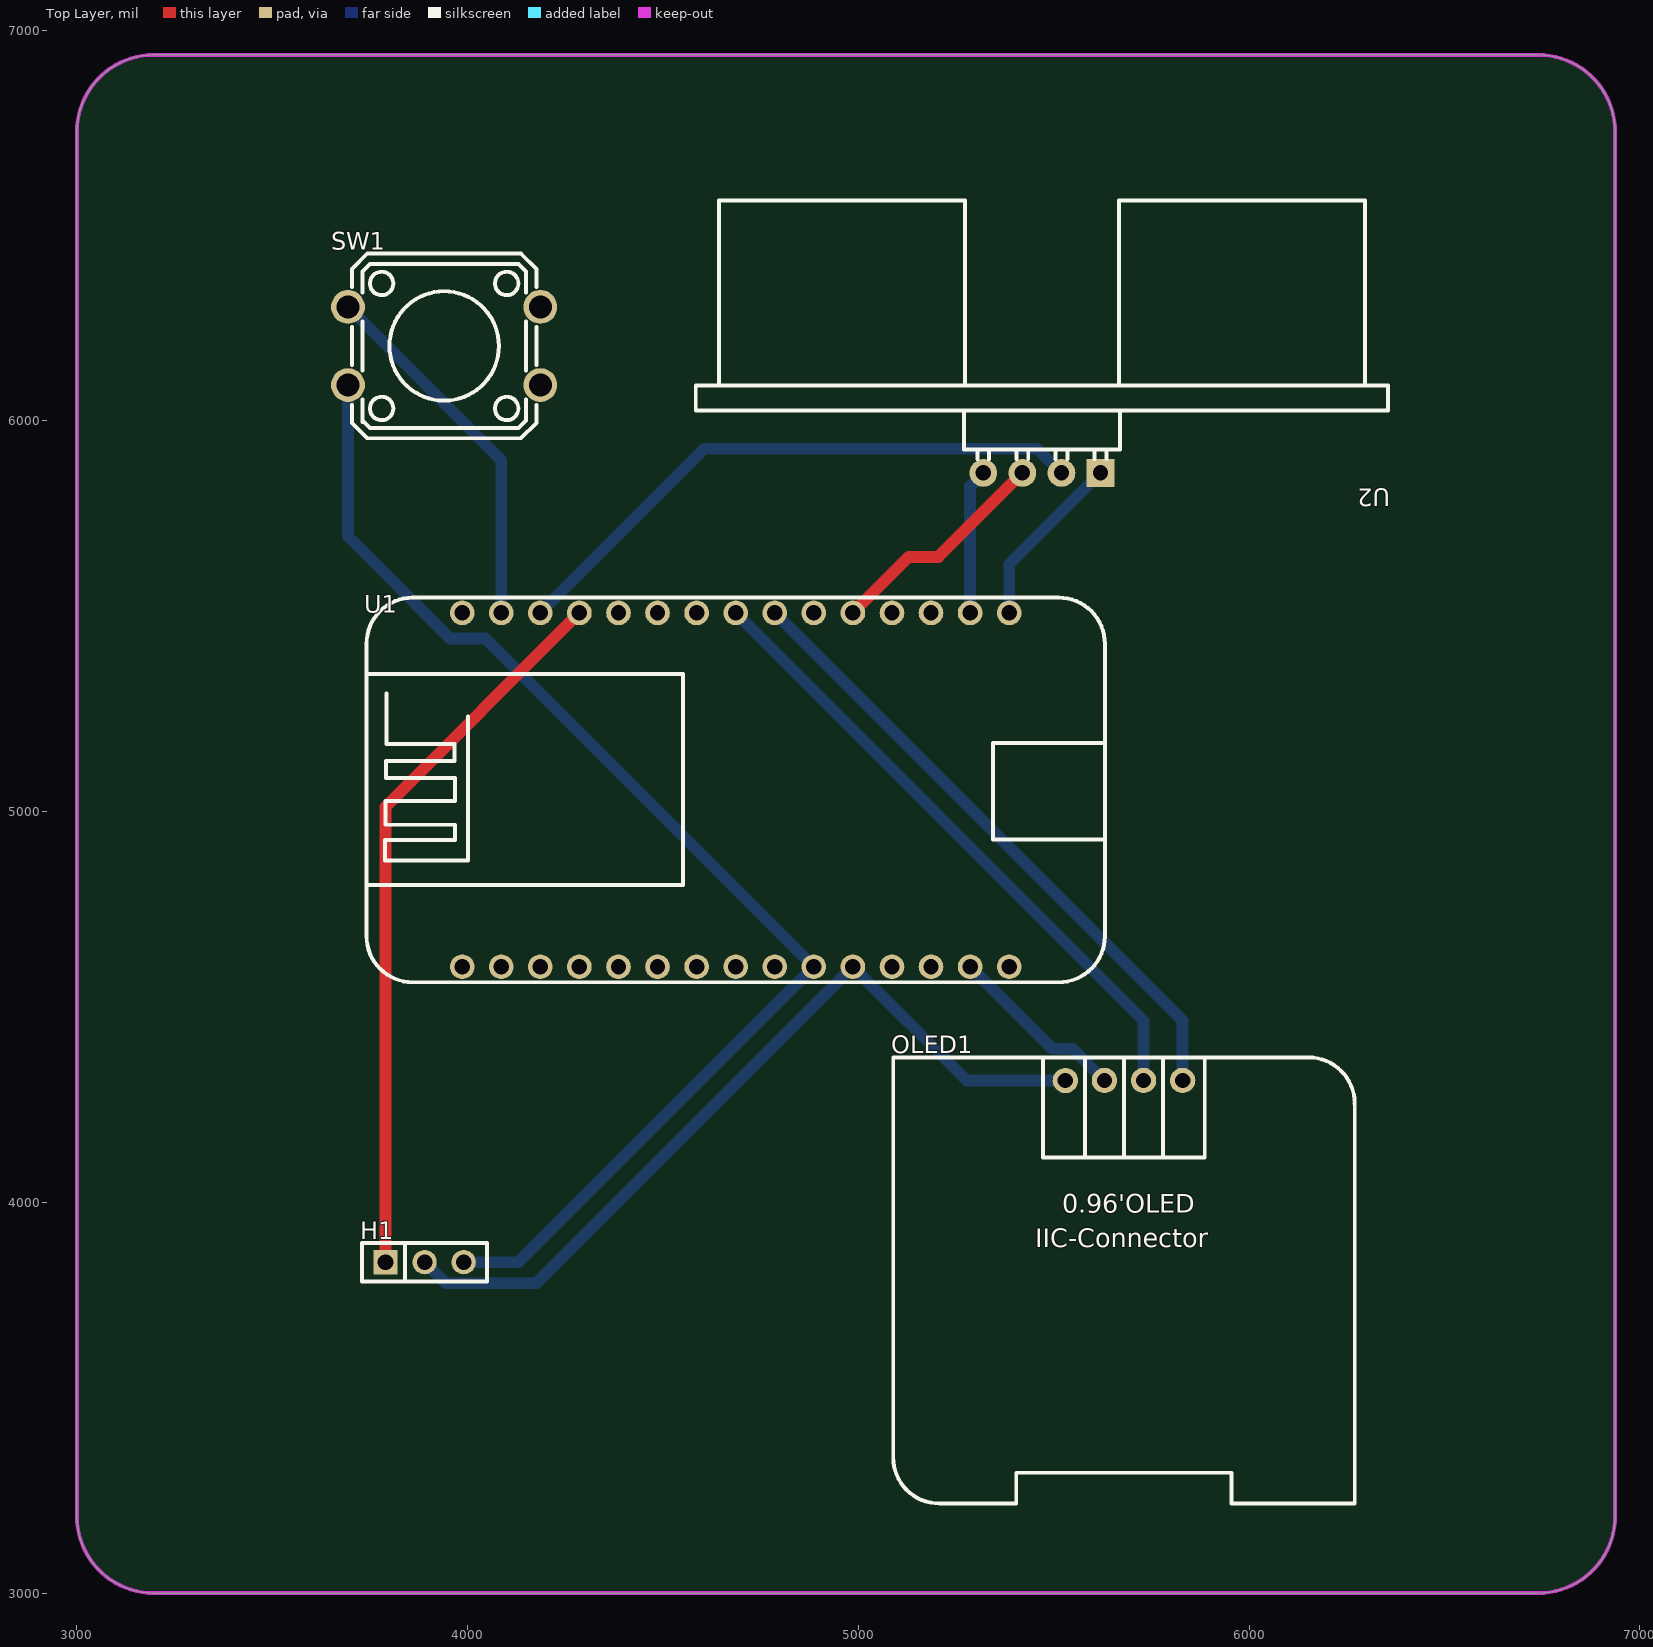
[diagram p0: Top Layer view]
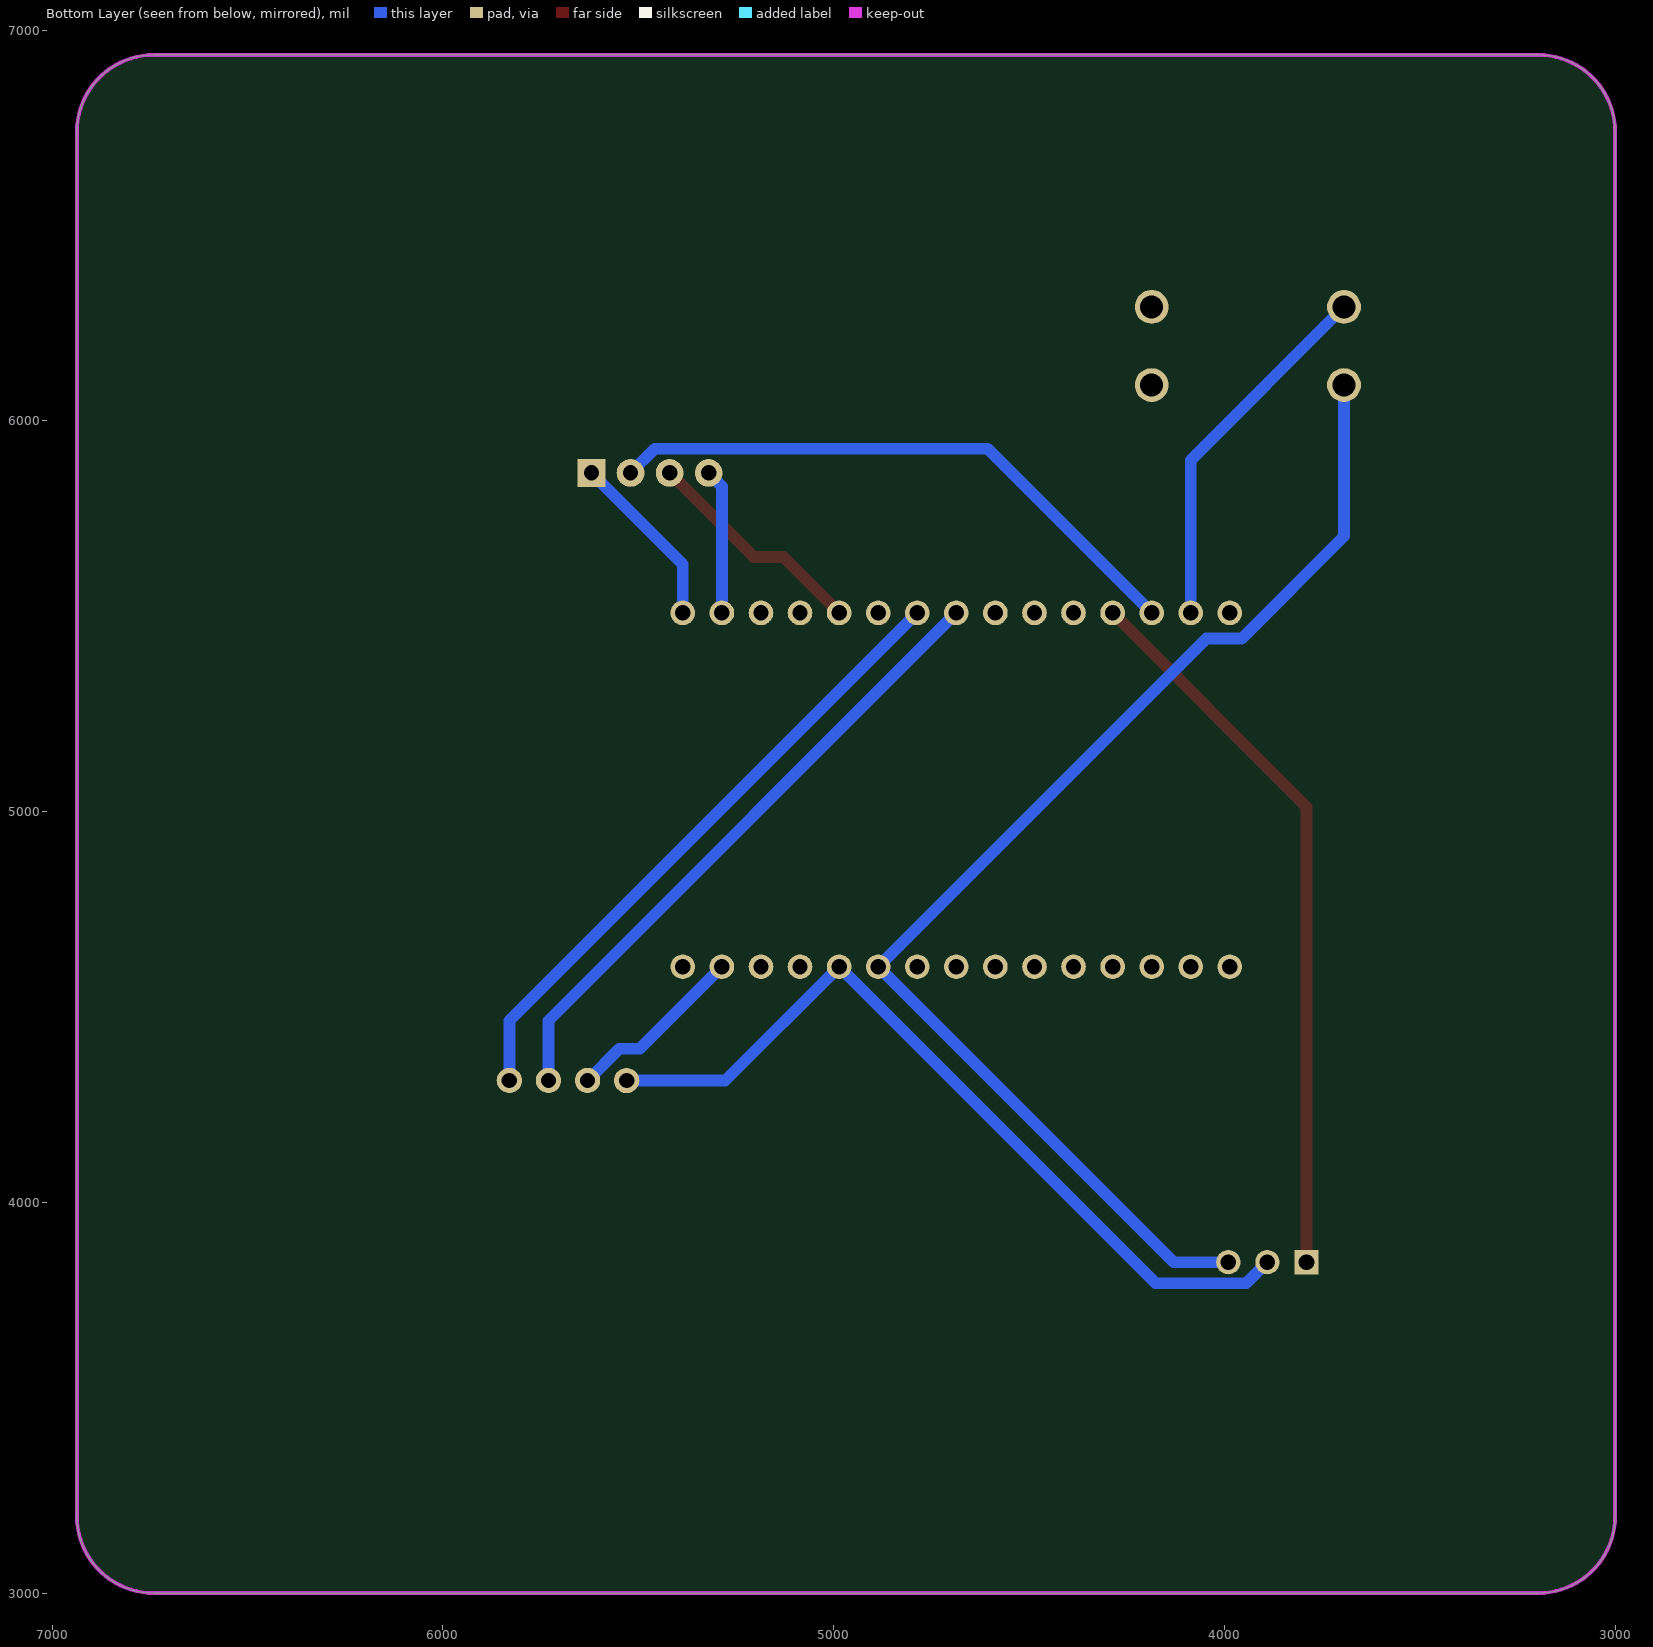
[diagram p1: Bottom Layer view, seen from below]
# Altium PCB MISC89069.pcbdoc
Units mil, origin at the board's own origin, x right, y up, seen from the top; angles counter-clockwise.
Board outline 3937.01 x 3937.01 mil, 2 copper layers (Top Layer, Bottom Layer), stack 62.206 mil thick; 5 components, 11 nets, 45 pads, 0 vias.

## Layer stack, top to bottom
Top Solder Mask Layer: solder mask 0.394, Dk 3.3
Top Layer: signal copper 1.379
Dielectric1: surface 59.449, FR4, Dk 4.5
Bottom Layer: signal copper 1.378
Bottom Solder Mask Layer: solder mask 0.394, Dk 3.3

## Board outline
3196.85,6937.01 ccw(c3196.85,6740.16) 3000,6740.16 3000,3196.85 ccw(c3196.85,3196.85) 3196.85,3000 6740.16,3000 ccw(c6740.16,3196.85) 6937.01,3196.85 6937.01,6740.16 ccw(c6740.16,6740.16) 6740.16,6937.01 3196.85,6937.01

## Design rules (kind name [scope] priority, off if disabled: settings)
BoardOutlineClearance copperThickness2oz_1 [All] p2 off: genericclearance=7.99 ignorepadtopadclearanceinfootprint=FALSE except(0: Arc-SplitContinuation Track-SplitContinuation SMDPad-SplitContinuation THPad-SplitContinuation Via-SplitContinuation Fill-SplitContinuation Region-SplitContinuation Poly-SplitContinuation Text-SplitContinuation Hole-SplitContinuation; 5.98: Arc-CutoutEdge Track-CutoutEdge SMDPad-CutoutEdge THPad-CutoutEdge Via-CutoutEdge Text-CutoutEdge; 6.89: Hole-OutlineEdge Hole-CutoutEdge; 10: Poly-OutlineEdge Poly-CutoutEdge; 11.81: Arc-OutlineEdge Track-OutlineEdge SMDPad-OutlineEdge THPad-OutlineEdge Via-OutlineEdge Fill-OutlineEdge Region-OutlineEdge Text-OutlineEdge Fill-CutoutEdge Region-CutoutEdge)
BoardOutlineClearance Plane_innerPlane_1 [All] p4 off: genericclearance=4.02 ignorepadtopadclearanceinfootprint=FALSE except(0: Arc-SplitContinuation Track-SplitContinuation SMDPad-SplitContinuation THPad-SplitContinuation Via-SplitContinuation Fill-SplitContinuation Region-SplitContinuation Poly-SplitContinuation Text-SplitContinuation Hole-SplitContinuation; 5.98: Arc-CutoutEdge Track-CutoutEdge SMDPad-CutoutEdge THPad-CutoutEdge Via-CutoutEdge Text-CutoutEdge; 6.89: Hole-OutlineEdge Hole-CutoutEdge; 10: Poly-OutlineEdge Poly-CutoutEdge; 11.81: Arc-OutlineEdge Track-OutlineEdge SMDPad-OutlineEdge THPad-OutlineEdge Via-OutlineEdge Fill-OutlineEdge Region-OutlineEdge Text-OutlineEdge Fill-CutoutEdge Region-CutoutEdge)
BoardOutlineClearance Copper_copperRegion_1 [All] p6 off: genericclearance=4.02 ignorepadtopadclearanceinfootprint=FALSE except(0: Arc-SplitContinuation Track-SplitContinuation SMDPad-SplitContinuation THPad-SplitContinuation Via-SplitContinuation Fill-SplitContinuation Region-SplitContinuation Poly-SplitContinuation Text-SplitContinuation Hole-SplitContinuation; 5.98: Arc-CutoutEdge Track-CutoutEdge SMDPad-CutoutEdge THPad-CutoutEdge Via-CutoutEdge Text-CutoutEdge; 6.89: Hole-OutlineEdge Hole-CutoutEdge; 10: Poly-OutlineEdge Poly-CutoutEdge; 11.81: Arc-OutlineEdge Track-OutlineEdge SMDPad-OutlineEdge THPad-OutlineEdge Via-OutlineEdge Fill-OutlineEdge Region-OutlineEdge Text-OutlineEdge Fill-CutoutEdge Region-CutoutEdge)
BoardOutlineClearance copperThickness1oz_1 [All] p8: genericclearance=4.02 ignorepadtopadclearanceinfootprint=FALSE except(0: Arc-SplitContinuation Track-SplitContinuation SMDPad-SplitContinuation THPad-SplitContinuation Via-SplitContinuation Fill-SplitContinuation Region-SplitContinuation Poly-SplitContinuation Text-SplitContinuation Hole-SplitContinuation; 5.98: Arc-CutoutEdge Track-CutoutEdge SMDPad-CutoutEdge THPad-CutoutEdge Via-CutoutEdge Text-CutoutEdge; 6.89: Hole-OutlineEdge Hole-CutoutEdge; 10: Poly-OutlineEdge Poly-CutoutEdge; 11.81: Arc-OutlineEdge Track-OutlineEdge SMDPad-OutlineEdge THPad-OutlineEdge Via-OutlineEdge Fill-OutlineEdge Region-OutlineEdge Text-OutlineEdge Fill-CutoutEdge Region-CutoutEdge)
Clearance copperThickness2oz [All] p1 off: gap=7.99 ignorepadtopadclearanceinfootprint=FALSE except(5.98: SMDPad-Track SMDPad-SMDPad THPad-Track SMDPad-THPad THPad-THPad Track-Via SMDPad-Via THPad-Via Via-Via Fill-SMDPad Region-SMDPad Fill-THPad Region-THPad Fill-Via Region-Via Fill-Fill Fill-Region Region-Region Arc-Track Arc-SMDPad Arc-THPad Arc-Via Fill-Arc Region-Arc Arc-Arc Text-Track SMDPad-Text Text-THPad Text-Via Fill-Text Region-Text Arc-Text Text-Text; 6.89: Hole-Track Hole-SMDPad Hole-THPad Hole-Via Fill-Hole Region-Hole Hole-Arc Hole-Text; 10: Poly-Track Poly-SMDPad Poly-THPad Poly-Via Poly-Fill Poly-Region Poly-Poly Poly-Arc Poly-Text Poly-Hole; 11.81: Fill-Track Region-Track)
Clearance Plane_innerPlane [All] p3 off: gap=4.02 ignorepadtopadclearanceinfootprint=FALSE except(5.98: SMDPad-Track SMDPad-SMDPad THPad-Track SMDPad-THPad THPad-THPad Track-Via SMDPad-Via THPad-Via Via-Via Fill-SMDPad Region-SMDPad Fill-THPad Region-THPad Fill-Via Region-Via Fill-Fill Fill-Region Region-Region Arc-Track Arc-SMDPad Arc-THPad Arc-Via Fill-Arc Region-Arc Arc-Arc Text-Track SMDPad-Text Text-THPad Text-Via Fill-Text Region-Text Arc-Text Text-Text; 6.89: Hole-Track Hole-SMDPad Hole-THPad Hole-Via Fill-Hole Region-Hole Hole-Arc Hole-Text; 10: Poly-Track Poly-SMDPad Poly-THPad Poly-Via Poly-Fill Poly-Region Poly-Poly Poly-Arc Poly-Text Poly-Hole; 11.81: Fill-Track Region-Track)
Clearance Copper_copperRegion [All] p5 off: gap=4.02 ignorepadtopadclearanceinfootprint=FALSE except(5.98: SMDPad-Track SMDPad-SMDPad THPad-Track SMDPad-THPad THPad-THPad Track-Via SMDPad-Via THPad-Via Via-Via Fill-SMDPad Region-SMDPad Fill-THPad Region-THPad Fill-Via Region-Via Fill-Fill Fill-Region Region-Region Arc-Track Arc-SMDPad Arc-THPad Arc-Via Fill-Arc Region-Arc Arc-Arc Text-Track SMDPad-Text Text-THPad Text-Via Fill-Text Region-Text Arc-Text Text-Text; 6.89: Hole-Track Hole-SMDPad Hole-THPad Hole-Via Fill-Hole Region-Hole Hole-Arc Hole-Text; 10: Poly-Track Poly-SMDPad Poly-THPad Poly-Via Poly-Fill Poly-Region Poly-Poly Poly-Arc Poly-Text Poly-Hole; 11.81: Fill-Track Region-Track)
Clearance copperThickness1oz [All] p7: gap=4.02 ignorepadtopadclearanceinfootprint=FALSE except(5.98: SMDPad-Track SMDPad-SMDPad THPad-Track SMDPad-THPad THPad-THPad Track-Via SMDPad-Via THPad-Via Via-Via Fill-SMDPad Region-SMDPad Fill-THPad Region-THPad Fill-Via Region-Via Fill-Fill Fill-Region Region-Region Arc-Track Arc-SMDPad Arc-THPad Arc-Via Fill-Arc Region-Arc Arc-Arc Text-Track SMDPad-Text Text-THPad Text-Via Fill-Text Region-Text Arc-Text Text-Text; 6.89: Hole-Track Hole-SMDPad Hole-THPad Hole-Via Fill-Hole Region-Hole Hole-Arc Hole-Text; 10: Poly-Track Poly-SMDPad Poly-THPad Poly-Via Poly-Fill Poly-Region Poly-Poly Poly-Arc Poly-Text Poly-Hole; 11.81: Fill-Track Region-Track)
DiffPairsRouting differentialPair [All] p1: maxlimit=6 minlimit=6 mostfreqgap=6 toplayer_minwidth=5 toplayer_prefwidth=10 toplayer_maxwidth=100 toplayer_mingap=6 toplayer_prefgap=6 toplayer_maxgap=6 bottomlayer_minwidth=5 bottomlayer_prefwidth=10 bottomlayer_maxwidth=100 bottomlayer_mingap=6 bottomlayer_prefgap=6 bottomlayer_maxgap=6 maxuncoupledlength=10
HoleToHoleClearance otherClearance [All] p1: gap=11.81 allowstackedmicrovias=TRUE
Length netLength [All] p1: minlimit=0 maxlimit=0
PasteMaskExpansion pasteMaskExpansion [All] p1: expansion=0
PlaneConnect innerPlane [All] p1: planeconnectstyle=Relief reliefexpansion=20 reliefentries=4 reliefconductorwidth=10 reliefairgap=10
PolygonConnect copperRegion [All] p1: connectstyle=Relief reliefconductorwidth=10 reliefentries=4 polygonreliefangle="90 Angle" airgapwidth=10 via.connectstyle=Relief via.reliefconductorwidth=10 via.reliefentries=4 via.polygonreliefangle="90 Angle" via.airgapwidth=10
RoutingVias viaSize [All] p1: holewidth=12.01 width=24.02 viastyle="Through Hole" minholewidth=11.81 minwidth=19.68 maxholewidth=248.03 maxwidth=393.7
SolderMaskExpansion solderMaskExpansion [IsVia] p1: expansion=-1000 istentingtop=TRUE
SolderMaskExpansion solderMaskExpansion [All] p2: expansion=2.01 istentingtop=FALSE
Width copperThickness2oz_2 [All] p1 off: maxlimit=100 minlimit=8 preferedwidth=10
Width copperThickness1oz_2 [All] p2: maxlimit=100 minlimit=5 preferedwidth=30

## Components (designator, comment, footprint, x,y, rotation, side; value= is the part's Value field where it differs from the comment)
H1 "" HDR-TH_3P-P2.54-V-F 3890,3847.01 r0 top
OLED1 "" 0.96OLED_4P 5680,4312.01 r0 top
SW1 "Tactile switch, 12*12*6 plastic head, 260G, travel 0.25mm, through-hole" KEY-TH_4P-L12.0-W12.0-P5.00-LS12.5 3940,6192.01 r0 top
U1 "STM32F103C8T6-Card" CONN-TH_L53.3-W22.9_STM32F103C8T6-CARD 4685,5047.01 r0 top
U2 "HC-SR04" TH_HC-SR04V 5470,5867.01 r180 top

## Footprints (in the part's own frame and the unit in brackets; to place one, negate y for a bottom-side part, rotate by r counter-clockwise, add the part's x,y. Pads: shape width x height; smd on the part's side, far side on the other; paste and mask are expansions set on the pad)
0.96OLED_4P [mm]
  round 1.65 hole 1 copper offset 0,0: 1(-3.81,-0.001) 2(-1.27,0.002) 3(1.27,0.002) 4(3.81,0.002)
  silkscreen extent -15,-27.5 15,1.5
CONN-TH_L53.3-W22.9_STM32F103C8T6-CARD [mm]
  round 1.6 hole 1: 1(-17.751,-11.273) 2(-15.211,-11.273) 3(-12.671,-11.273) 4(-10.131,-11.273) 5(-7.591,-11.273) 6(-5.051,-11.273) 7(-2.511,-11.273) 8(0.029,-11.273) 9(2.569,-11.273) 10(5.109,-11.273) 11(7.649,-11.273) 12(10.189,-11.273) 13(12.729,-11.273) 14(15.269,-11.273) 15(17.809,-11.273) 16(17.809,11.727) 17(15.269,11.727) 18(12.729,11.727) 19(10.189,11.727) 20(7.649,11.727) 21(5.109,11.727) 22(2.569,11.727) 23(0.029,11.727) 24(-2.511,11.727) 25(-5.051,11.727) 26(-7.591,11.727) 27(-10.131,11.727) 28(-12.671,11.727) 29(-15.211,11.727) 30(-17.751,11.727)
  silkscreen extent -23.97,-12.28 24.03,12.72
HDR-TH_3P-P2.54-V-F [mil]
  rect 62x62 hole 40.16: 1(-100,0)
  round 62 hole 40.16: 2(0,0) 3(100,0)
  silkscreen extent -160,-49 160,49
KEY-TH_4P-L12.0-W12.0-P5.00-LS12.5 [mm]
  round 2.2 hole 1.5: 1(-6.251,2.54) 2(6.251,2.54) 3(-6.251,-2.54) 4(6.251,-2.54)
  silkscreen extent -5.99,-6 5.99,6
TH_HC-SR04V [mm]
  rect 1.8x1.8 hole 1.001: 1(-3.81,0)
  round 1.8 hole 1.001: 2(-1.27,0) 3(1.27,0) 4(3.81,0)
  silkscreen extent -22.5,-17.7 22.5,-0.89

## Nets (pads, with @x,y where several pads share a name; then routed paths per layer and width w, separated by ;. In a path a pad name is that pad's centre, name@x,y a point inside that pad or via, vN(x,y) a via of type N, cw(c..) or ccw(c..) an arc to the next point about the centre after c; other vN are vias at no path point)
$1N395: OLED1.2 U1.14 | length 464.4
  Bottom Layer w30: U1.14@5286.15,4603.19 5496.15,4393.19 5548.87,4393.19 OLED1.2
$1N529: H1.2 OLED1.1 U1.11 | length 2118.4
  Bottom Layer w30: H1.2 3943.82,3793.19 4176.15,3793.19 4986.15,4603.19 5277.38,4311.96 OLED1.1
$1N541: H1.3 SW1.3 U1.10 | length 3244.8
  Bottom Layer w30: SW1.3 3693.9,5705.44 3956.15,5443.19 4046.15,5443.19 4886.15,4603.19 4129.97,3847.01 H1.3
$1N625: H1.1 U1.27 | length 1867.2
  Top Layer w30: H1.1 3790,5012.55 U1.27
$1N700: U1.16 U2.1 | length 455.2
  Bottom Layer w30: U1.16@5386.15,5508.7 5386.15,5633.16 U2.1
$1N706: U1.17 U2.4 | length 372.3
  Bottom Layer w30: U1.17@5286.15,5508.7 5286.15,5833.16 U2.4
$1N719: U1.20 U2.3 | length 582.3
  Top Layer w30: U1.20@4986.15,5508.7 5129.46,5652.01 5205,5652.01 U2.3
$1N729: OLED1.4 U1.22 | length 1629
  Bottom Layer w30: U1.22 5830,4464.85 OLED1.4
$1N739: OLED1.3 U1.23 | length 1629
  Bottom Layer w30: U1.23 5730,4464.85 OLED1.3
$1N749: U1.28 U2.2 | length 1533.4
  Bottom Layer w30: U1.28 4606.15,5928.7 5458.31,5928.7 U2.2
$1N758: SW1.1 U1.29 | length 945.8
  Bottom Layer w30: SW1.1 4086.15,5899.76 U1.29
pads on no net: SW1.2 SW1.4 U1.1 U1.2 U1.3 U1.4 U1.5 U1.6 U1.7 U1.8 U1.9 U1.12 U1.13 U1.15 U1.18 U1.19 U1.21 U1.24 U1.25 U1.26 U1.30

## Keep-outs
Board Outline Layer:
  the board outline again, w10